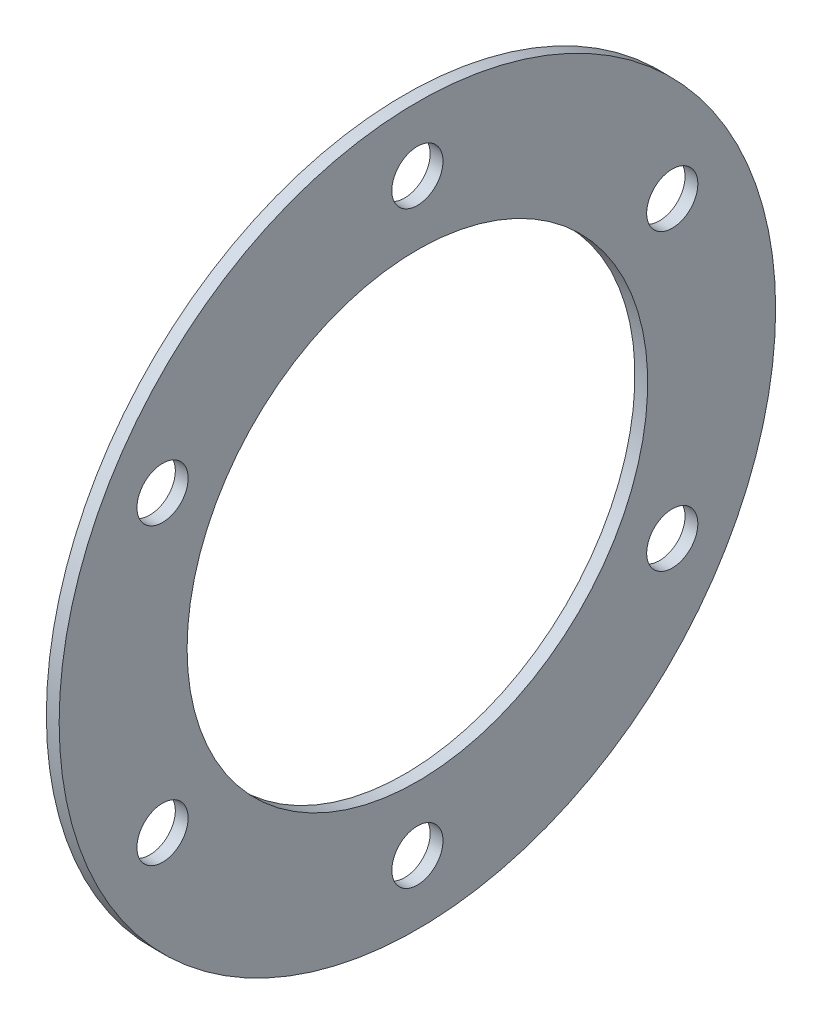
from build123d import *

# Parameters (mm, degrees)
SKETCH1_W          = 2
SKETCH1_H          = 20
SKETCH2_R          = 4
CUT_EXTRUDE1_DEPTH = 10
SCALE_1_SCALE      = 1.875


with BuildPart() as part:
    # Sketch1 → Revolve1 (revolve)
    with BuildSketch(Plane.XY, mode=Mode.PRIVATE) as revolve1_sk:
        with Locations((1, 46)):
            Rectangle(SKETCH1_W, SKETCH1_H)
    revolve(revolve1_sk.sketch.rotate(Axis((0, 0, 0), (1, 0, 0)), 90), axis=Axis((0, 0, 0), (1, 0, 0)))

    # Sketch2 → Cut-Extrude1 (cut)
    with BuildSketch(Plane(origin=(2, 0, 0), x_dir=(0, 0, -1), z_dir=(1, 0, 0))):
        with Locations((0, 46)):
            Circle(SKETCH2_R)
        with Locations((39.837168574, 23)):
            Circle(SKETCH2_R)
        with Locations((-39.837168574, 23)):
            Circle(SKETCH2_R)
        with Locations((-39.837168574, -23)):
            Circle(SKETCH2_R)
        with Locations((0, -46)):
            Circle(SKETCH2_R)
        with Locations((39.837168574, -23)):
            Circle(SKETCH2_R)
    extrude(amount=-CUT_EXTRUDE1_DEPTH, mode=Mode.SUBTRACT)


with BuildPart() as part_1:
    # Scale 1: scaled about (1, 0, 0)
    add(part.part.scale(SCALE_1_SCALE).moved(Location((-0.875, 0, 0))))


solid = part_1.part
